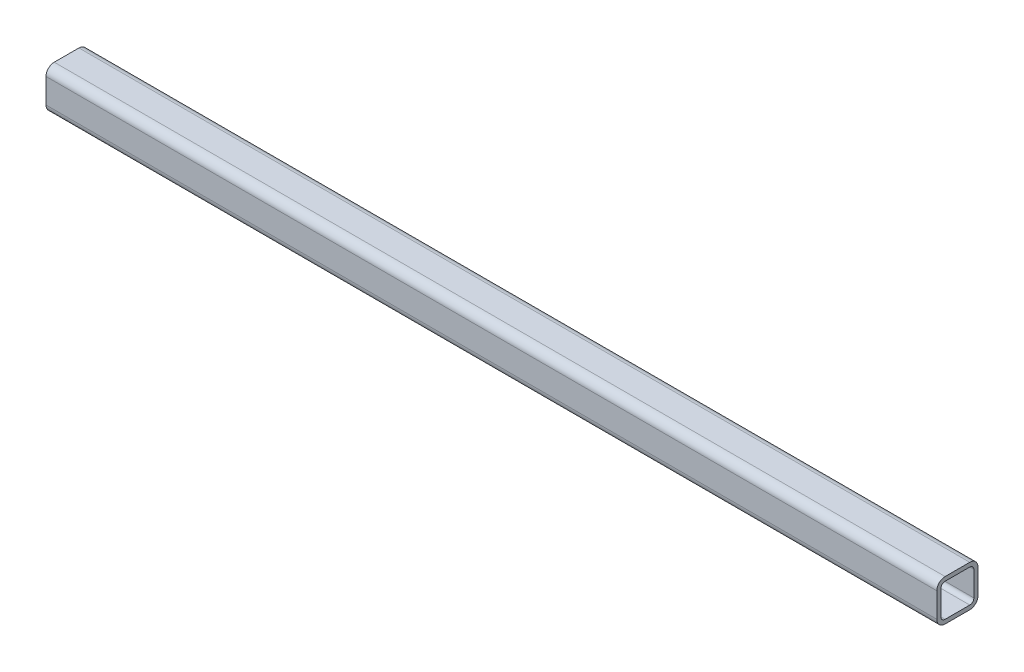
SolidWorks part; units mm, degrees
ref_plane "前视基准面" through (0, 0, 0) normal (0, 0, 1) x (1, 0, 0)
ref_plane "上视基准面" through (0, 0, 0) normal (0, 1, 0) x (1, 0, 0)
ref_plane "右视基准面" through (0, 0, 0) normal (1, 0, 0) x (0, 0, -1)
sketch "草图1" plane through (0, 0, 0) normal (0, 1, 0) x (1, 0, 0)
  line L0 (-433, 0) -> (433, 0)
  line L1 (-627, 0) -> (627, 0) construction
  point P5 (0, 0)
  dimension "D1" = 866
other "Gb／6728-1986方形空心型钢 040 X 40 X 4(1)"
ref_plane "基准面1" through (-433, 0, 0) normal (1, 0, 0) x (0, 0, -1)
sketch "Sketch1" plane through (-433, 0, 0) normal (1, 0, 0) x (0, 0, -1)
  line L0 (-12, -16) -> (12, -16)
  line L1 (-16, -12) -> (-16, 12)
  line L2 (12, 16) -> (-12, 16)
  line L3 (16, 12) -> (16, -12)
  line L4 (-12, -20) -> (12, -20)
  line L5 (-20, -12) -> (-20, 12)
  line L6 (12, 20) -> (-12, 20)
  line L7 (20, 12) -> (20, -12)
  arc A0 (20, 12) -> (12, 20) centre (12, 12) ccw
  arc A1 (12, -20) -> (20, -12) centre (12, -12) ccw
  arc A2 (-20, -12) -> (-12, -20) centre (-12, -12) ccw
  arc A3 (-12, 20) -> (-20, 12) centre (-12, 12) ccw
  arc A4 (-12, 16) -> (-16, 12) centre (-12, 12) ccw
  arc A5 (16, 12) -> (12, 16) centre (12, 12) ccw
  arc A6 (12, -16) -> (16, -12) centre (12, -12) ccw
  arc A7 (-16, -12) -> (-12, -16) centre (-12, -12) ccw
  point P0 (-20, 0)
  point P1 (20, 0)
  point P2 (0, 20)
  point P3 (0, -20)
  point P4 (0, 0)
  point P5 (-20, -20)
  point P6 (20, -20)
  point P7 (20, 20)
  point P8 (-20, 20)
  point P33 (0, 0)
  dimension "D1" = 8
  dimension "Thickness" = 4
  dimension "V_leg" = 40
